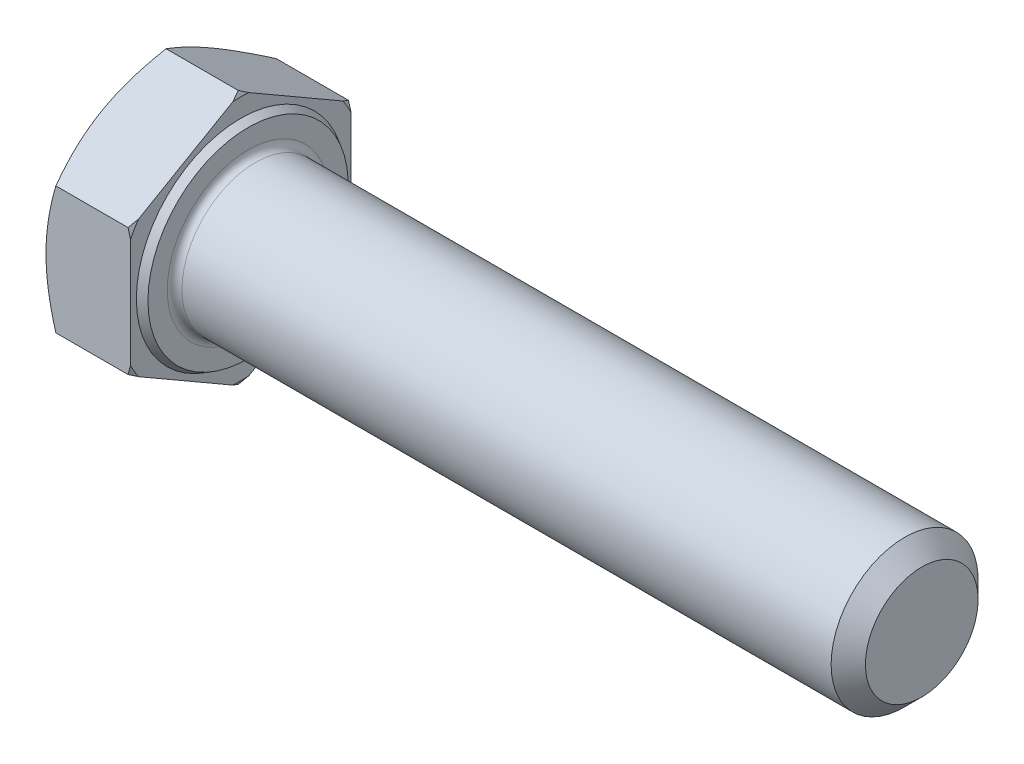
SolidWorks part; units mm, degrees
material "Steel"
ref_plane "Front" through (0, 0, 0) normal (0, 0, 1) x (1, 0, 0)
ref_plane "Top" through (0, 0, 0) normal (0, 1, 0) x (1, 0, 0)
ref_plane "Right" through (0, 0, 0) normal (1, 0, 0) x (0, 0, -1)
sketch "Dimension Sketch" plane through (0, 0, 0) normal (0, 0, 1) x (1, 0, 0)
  line L0 (0, 0) -> (30, 0) construction
  line L1 (0, 0) -> (0, 12) construction
  point P3 (1.75, 0)
  point P4 (0.6, 0)
  point P6 (0, 14.7)
  point P7 (0, 12.7)
  point P8 (0, 16.47)
  point P9 (19.85, 0)
  point P10 (7.5, 0)
  point P11 (4.94, 0)
  point P12 (0.6, 0)
  point P13 (18, 0)
  point P14 (55, 0)
  point P15 (25, 0)
  point P16 (46.25, 0)
  dimension "b(参考)" = 30
  dimension "P" = 1.75
  dimension "d" = 12
  dimension "c(max)" = 0.6
  dimension "da(max)" = 14.7
  dimension "ds(max)" = 12.7
  dimension "dw(min)" = 16.47
  dimension "e(min)" = 19.85
  dimension "k(公称)" = 7.5
  dimension "kw(min)" = 4.94
  dimension "r(min)" = 0.6
  dimension "s(公称)" = 18
  dimension "l" = 55
  dimension "lg(max)" = 25
  dimension "ls(min)" = 16.25
sketch "Sketch1" plane through (0, 0, 0) normal (1, 0, 0) x (0, 0, -1)
  line L0 (9, 5.1962) -> (9, -5.1962)
  line L1 (-9, 5.1962) -> (-9, -5.1962)
  line L2 (9, -5.1962) -> (0, -10.3923)
  line L3 (0, -10.3923) -> (-9, -5.1962)
  line L4 (9, 5.1962) -> (0, 10.3923)
  line L5 (0, 10.3923) -> (-9, 5.1962)
  point P6 (0, 9.4577)
  dimension "D1" = 19.85
  dimension "s" = 18
  dimension "D2" = 120
  dimension "D3" = 9
  dimension "D4" = 9
  dimension "D5" = 9
extrude "Boss-Extrude" add sketch "Sketch1" along normal blind 7.5
sketch "Sketch2" plane through (0, 0, 0) normal (0, 0, 1) x (1, 0, 0)
  line L0 (0, 5.1962) -> (0, -5.1962) construction
  line L1 (0, 0) -> (62.5, 0)
  line L2 (0, 0) -> (0, 6)
  line L3 (0, 6) -> (7.5, 6)
  line L4 (62.5, 0) -> (62.5, 4.4845)
  line L5 (7.5, 10.3923) -> (7.5, 5.1962) construction
  line L7 (0, 0) -> (-51.1435, 0) construction
  line L8 (62.5, -4.4845) -> (7.5, -6) construction
  line L9 (0, -6) -> (7.5, -6) construction
  line L10 (9.25, 6) -> (9.25, 0) construction
  line L11 (32.5, 6) -> (32.5, 0) construction
  line L12 (7.5, 5.1962) -> (7.5, -5.1962) construction
  line L13 (7.5, 6) -> (62.5, 6)
  line L14 (62.5, 6) -> (62.5, 4.4845)
  dimension "l" = 55
  dimension "d" = 12
  dimension "Minor_dia" = 8.969
  dimension "p" = 1.75
  dimension "b" = 30
revolve "Boss-Revolve1" add sketch "Sketch2" angle 360 about L7
cosmetic thread "Cosmetic Thread1" parameters "D1"=30, "D2"=9.6
sketch "Sketch3" plane through (0, 0, 0) normal (0, 0, 1) x (1, 0, 0)
  line L0 (0, 9) -> (3.6906, 15.3923)
  line L1 (0, 10.3923) -> (0, 5.1962) construction
  line L2 (3.6906, 15.3923) -> (3.6906, 20.3923)
  line L3 (3.6906, 20.3923) -> (-10, 20.3923)
  line L4 (-10, 20.3923) -> (-10, 9)
  line L5 (-10, 9) -> (0, 9)
  line L6 (0, 0) -> (99.06, 0) construction
  line L7 (7.5, 10.3923) -> (0, 10.3923) construction
  dimension "D1" = 9
  dimension "D2" = 5
  dimension "D3" = 10
  dimension "D4" = 5
  dimension "Head_ch_ang" = 30
revolve "Cut-Revolve1" cut sketch "Sketch3" angle 360 about L6
sketch "Sketch5" plane through (0, 0, 0) normal (0, 0, 1) x (1, 0, 0)
  line L0 (7.5, 9) -> (3.8094, 15.3923)
  line L1 (7.5, 10.3923) -> (7.5, 5.1962) construction
  line L2 (3.8094, 15.3923) -> (3.8094, 20.3923)
  line L3 (3.8094, 20.3923) -> (13.8094, 20.3923)
  line L4 (13.8094, 20.3923) -> (13.8094, 9)
  line L5 (13.8094, 9) -> (7.5, 9)
  line L7 (7.5, 10.3923) -> (0.8038, 10.3923) construction
  line L8 (0, 0) -> (99.06, 0) construction
  line L9 (0, 0) -> (99.06, 0) construction
  dimension "D1" = 9
  dimension "D2" = 5
  dimension "D3" = 10
  dimension "Head_ch_ang" = 30
  dimension "D4" = 5
revolve "Cut-Revolve2" cut sketch "Sketch5" angle 360 about L8
sketch "Sketch4" plane through (0, 0, 0) normal (0, 0, 1) x (1, 0, 0)
  line L0 (7.4, 8.235) -> (7.4, 0) construction
  line L1 (7.5, 10.3923) -> (7.5, 5.1962) construction
  line L2 (7.5, 8.1773) -> (6.9, 8.5237)
  line L3 (7.5, 8.1773) -> (7.5, 20.3923)
  line L4 (7.5, 20.3923) -> (6.9, 20.3923)
  line L5 (0, 0) -> (95.25, 0) construction
  line L6 (-51.1435, 0) -> (0, 0) construction
  line L7 (6.9, 8.5237) -> (6.9, 20.3923)
  line L8 (6.6962, 10.3923) -> (0.8038, 10.3923) construction
  line L9 (7.5, 7.7942) -> (7.5, 9) construction
  line L10 (6.6962, 10.3923) -> (0.8038, 10.3923) construction
  point P15 (2.46, 10.3923)
  dimension "D1" = 120
  dimension "D2" = 10
  dimension "D3" = 0.1
  dimension "c" = 0.6
  dimension "D4" = 16.47
  dimension "D5" = 4.94
revolve "Cut-Revolve3" cut sketch "Sketch4" angle 360 about L5
chamfer "Chamfer" distance 1.4 angle 45 1 edges at (62.5, 0, -6)
sketch "Sketch9" plane through (0, 0, 0) normal (0, 0, 1) x (1, 0, 0)
  line L0 (7.5, -8.1773) -> (7.5, 8.1773) construction
  line L1 (61.1, 6) -> (7.5, 6) construction
  line L2 (0, 0) -> (7.5, 0) construction
  line L3 (7.5, 6.6) -> (7.5, 6)
  line L4 (7.5, 6) -> (8.1, 6)
  arc A0 (7.5, 6.6) -> (8.1, 6) centre (8.1, 6.6) ccw
  dimension "D1" = 0.6
revolve "Revolve1" add sketch "Sketch9" angle 360 about L2
sketch "Sketch6" plane through (0, 0, 0) normal (0, 0, 1) x (1, 0, 0)
  line L0 (60.225, -4.4845) -> (59.3501, -6)
  line L1 (60.225, -4.4845) -> (61.1, -6)
  line L2 (61.1, -6) -> (61.1, -10.3923)
  line L3 (-3.175, 0) -> (0, 0) construction
  line L4 (61.1, -6) -> (61.1, 6) construction
  line L5 (61.1, -10.3923) -> (59.3501, -10.3923)
  line L6 (59.3501, -10.3923) -> (59.3501, -6)
  line L7 (8.1, -6) -> (61.1, -6) construction
  line L9 (6.6962, -10.3923) -> (0.8038, -10.3923) construction
  dimension "Thread_minor" = 8.969
  dimension "SideAngle" = 60
  dimension "VeeAngle" = 60
revolve "Cut-Revolve4" [suppressed] cut sketch "Sketch6" angle 360 about L3
pattern_linear "LPattern1" [suppressed]
